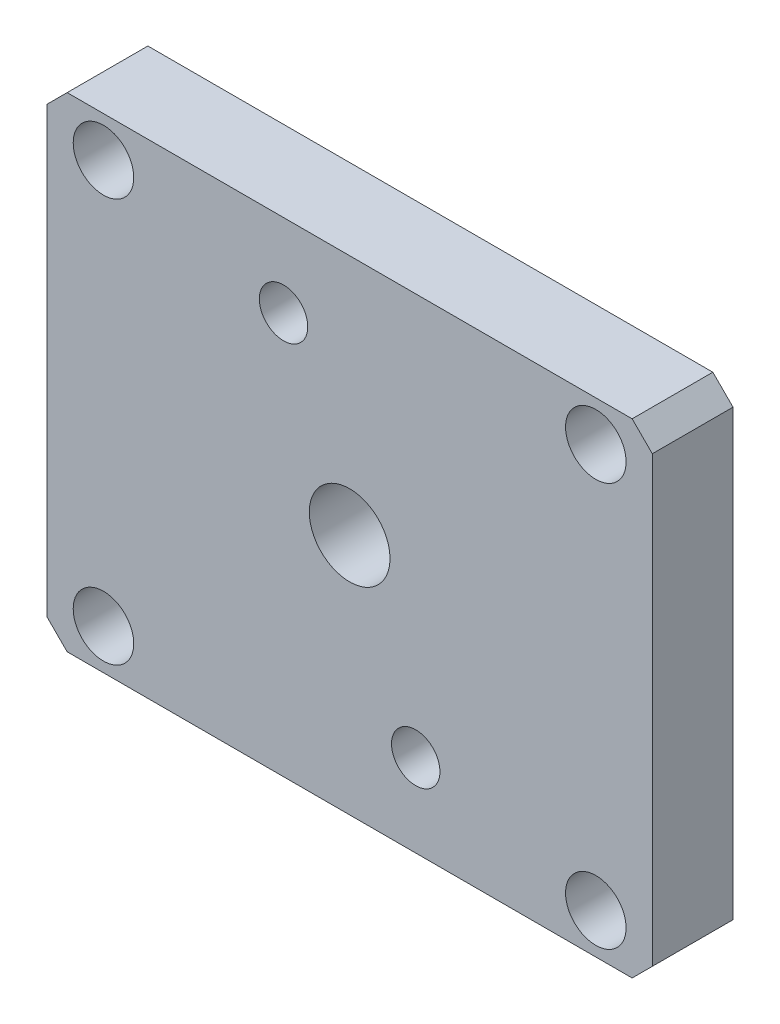
SolidWorks part; units mm, degrees
ref_plane "Front Plane" through (0, 0, 0) normal (0, 0, 1) x (1, 0, 0)
ref_plane "Top Plane" through (0, 0, 0) normal (0, 1, 0) x (1, 0, 0)
ref_plane "Right Plane" through (0, 0, 0) normal (1, 0, 0) x (0, 0, -1)
sketch "Sketch2" plane through (0, 0, 0) normal (0, 0, 1) x (1, 0, 0)
  line L0 (75, -55) -> (70, -60)
  line L1 (70, -60) -> (-70, -60)
  line L2 (75, -55) -> (75, 55)
  line L3 (70, 60) -> (-70, 60)
  line L4 (-75, -55) -> (-75, 55)
  line L5 (75, -60) -> (-75, 60) construction
  line L6 (75, 60) -> (-75, -60) construction
  line L7 (75, 55) -> (70, 60)
  line L8 (-75, 55) -> (-70, 60)
  line L9 (-70, -60) -> (-75, -55)
  point P0 (0, 0)
  dimension "D1" = 150
  dimension "D2" = 120
extrude "Boss-Extrude1" add sketch "Sketch2" along normal blind 20
sketch "Sketch3" plane through (0, 0, 0) normal (0, 0, -1) x (-1, 0, 0)
  line L0 (70, -60) -> (-70, -60) construction
  line L1 (75, 55) -> (75, -55) construction
  line L2 (75, 0) -> (0, 0) construction
  line L3 (0, 0) -> (0, -60) construction
  circle A0 centre (61, -50) radius 7.5
  circle A1 centre (61, 50) radius 7.5
  circle A2 centre (-61, -50) radius 7.5
  circle A3 centre (-61, 50) radius 7.5
  dimension "D1" = 15
  dimension "D3" = 14
  dimension "D2" = 10
extrude "Cut-Extrude1" cut sketch "Sketch3" against normal through all both and the other way through all
sketch "Sketch4" plane through (0, 0, 0) normal (0, 0, -1) x (-1, 0, 0)
  circle A0 centre (0, 0) radius 10
  dimension "D1" = 20
extrude "Cut-Extrude2" cut sketch "Sketch4" against normal blind 59
sketch "Sketch5" plane through (0, 0, 0) normal (0, 0, -1) x (-1, 0, 0)
  circle A0 centre (-16.3789, -39.542) radius 6
  circle A1 centre (-39.542, -16.3789) radius 6 construction
  circle A2 centre (-39.542, 16.3789) radius 6 construction
  circle A3 centre (-16.3789, 39.542) radius 6 construction
  circle A4 centre (16.3789, 39.542) radius 6
  circle A5 centre (39.542, 16.3789) radius 6 construction
  circle A6 centre (39.542, -16.3789) radius 6 construction
  circle A7 centre (16.3789, -39.542) radius 6 construction
  point P19 (0, 0)
  dimension "D1" = 12
  dimension "D2" = 8
extrude "Cut-Extrude3" cut sketch "Sketch5" against normal up to surface (20 mm away)
